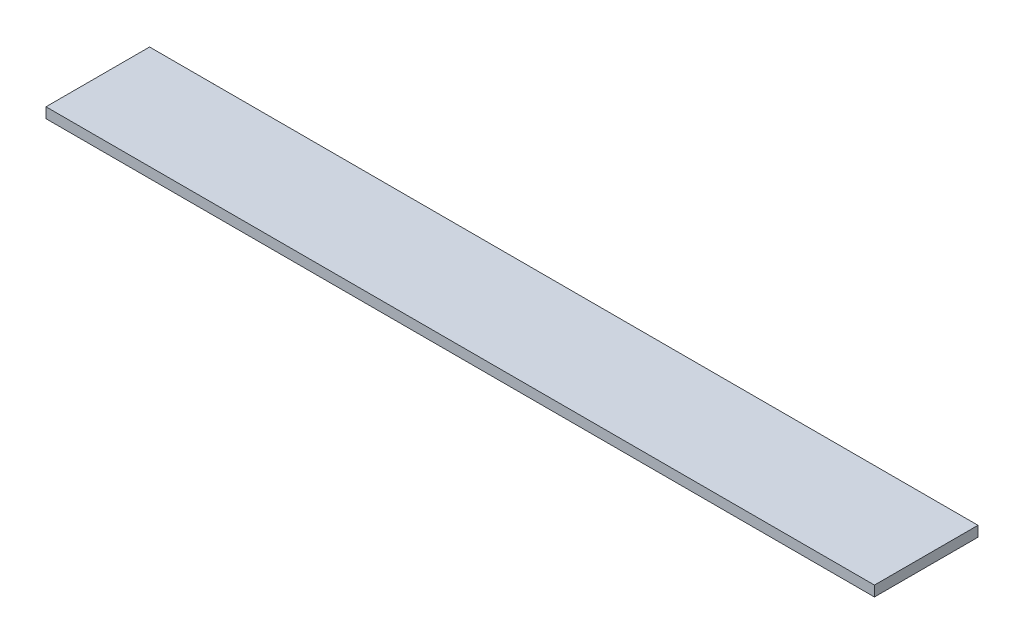
SolidWorks part; units mm, degrees
ref_plane "Front Plane" through (0, 0, 0) normal (0, 0, 1) x (1, 0, 0)
ref_plane "Top Plane" through (0, 0, 0) normal (0, 1, 0) x (1, 0, 0)
ref_plane "Right Plane" through (0, 0, 0) normal (1, 0, 0) x (0, 0, -1)
sketch "Sketch1" plane through (0, 0, 0) normal (0, 1, 0) x (1, 0, 0)
  line L1 (-200, 25) -> (200, 25)
  line L2 (-200, 25) -> (-200, -25)
  line L3 (-200, -25) -> (200, -25)
  line L4 (200, 25) -> (200, -25)
  line L5 (-200, 25) -> (200, -25) construction
  line L6 (-200, -25) -> (200, 25) construction
  point P0 (0, 0)
  dimension "D1" = 50
  dimension "D2" = 400
extrude "Boss-Extrude1" add sketch "Sketch1" along normal blind 5 contours L1 L4 L3 L2
